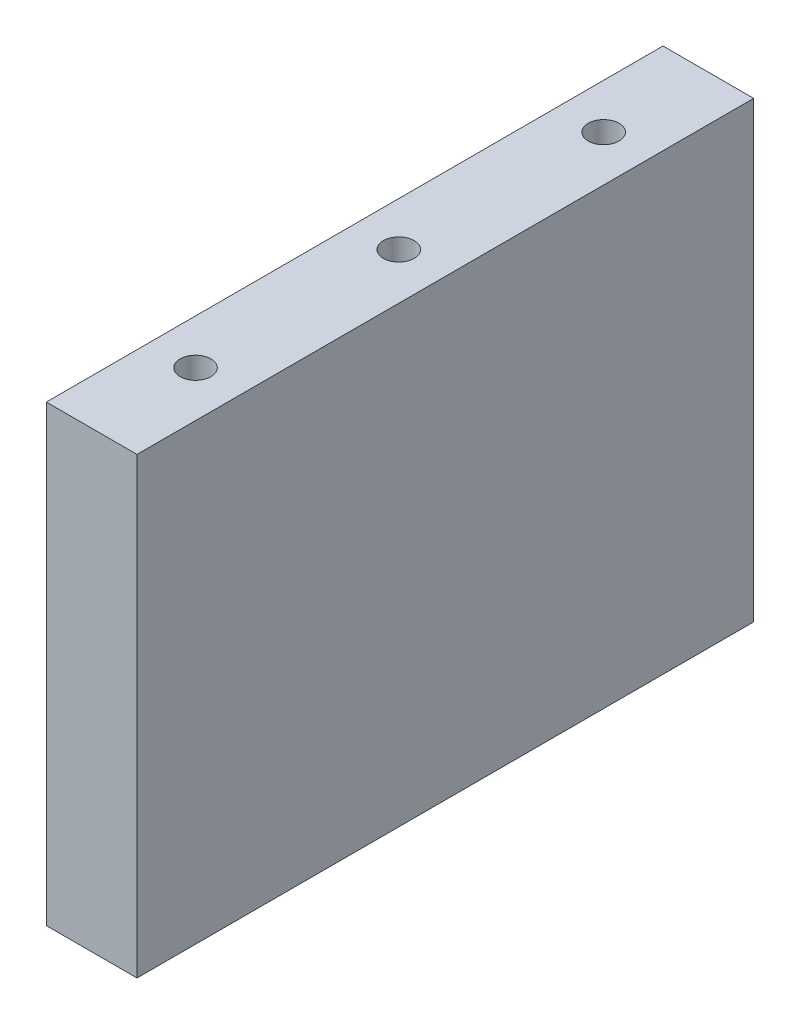
SolidWorks part; units mm, degrees
ref_plane "前视基准面" through (0, 0, 0) normal (0, 0, 1) x (1, 0, 0)
ref_plane "上视基准面" through (0, 0, 0) normal (0, 1, 0) x (1, 0, 0)
ref_plane "右视基准面" through (0, 0, 0) normal (1, 0, 0) x (0, 0, -1)
sketch "草图1" plane through (0, 0, 0) normal (1, 0, 0) x (0, 0, -1)
  line L1 (-68, 50) -> (68, 50)
  line L2 (-68, 50) -> (-68, -50)
  line L3 (-68, -50) -> (68, -50)
  line L4 (68, 50) -> (68, -50)
  line L5 (-68, 50) -> (68, -50) construction
  line L6 (-68, -50) -> (68, 50) construction
  point P0 (0, 0)
  dimension "D1" = 136
  dimension "D2" = 100
extrude "凸台-拉伸1" add sketch "草图1" along normal blind 20
hole_wizard "M8 螺纹孔1" positions "草图2" profile "草图3" tap size "M8" standard "GB"
sketch "草图2" plane through (0, 50, 0) normal (0, 1, 0) x (1, 0, 0)
  line L0 (0, 0) -> (31.5986, 0) construction
  line L2 (10, -68) -> (9.5475, 47.828) construction
  line L3 (20, -68) -> (0, -68) construction
  point P0 (9.9101, 45)
  point P2 (9.9101, -45)
  point P15 (9.7343, 0)
  dimension "D1" = 90
sketch "草图3" plane through (9.9101, 50, -45) normal (1, 0, 0) x (0, 0, 1)
  line L0 (0, 0) -> (0, 21.7929)
  line L1 (0, 21.7929) -> (3.4, 19.75)
  line L2 (3.4, 19.75) -> (3.4, 0)
  line L5 (3.4, 0) -> (0, 0)
  line L10 (0, 21.7929) -> (-3.4, 19.75) construction
  line L11 (0, -6.35) -> (0, 107.95) construction
  dimension "螺纹孔钻头直径" = 6.8
  dimension "螺纹孔钻头深度" = 19.75
  dimension "导头角度" = 118
cosmetic thread "孔螺蚊线1" parameters "D1"=16, "D2"=8
cosmetic thread "孔螺蚊线2" parameters "D1"=16, "D2"=8
cosmetic thread "孔螺蚊线6" parameters "D1"=16, "D2"=8
hole_wizard "M8 螺纹孔2" positions "草图4" profile "草图5" tap size "M8" standard "GB"
sketch "草图4" plane through (0, -50, 0) normal (0, -1, 0) x (-1, 0, 0)
  line L0 (-10, -68) -> (-10, 27.3351) construction
  line L1 (-20, -68) -> (0, -68) construction
  line L3 (0, 0) -> (-33.0288, 0) construction
  point P0 (-10, 45)
  point P2 (-10, 0)
  point P4 (-10, -45)
  dimension "D1" = 90
sketch "草图5" plane through (10, -50, -45) normal (1, 0, 0) x (0, 0, -1)
  line L0 (0, 0) -> (0, 21.7929)
  line L1 (0, 21.7929) -> (3.4, 19.75)
  line L2 (3.4, 19.75) -> (3.4, 0)
  line L5 (3.4, 0) -> (0, 0)
  line L10 (0, 21.7929) -> (-3.4, 19.75) construction
  line L11 (0, -6.35) -> (0, 107.95) construction
  dimension "螺纹孔钻头直径" = 6.8
  dimension "螺纹孔钻头深度" = 19.75
  dimension "导头角度" = 118
cosmetic thread "孔螺蚊线3" parameters "D1"=16, "D2"=8
cosmetic thread "孔螺蚊线4" parameters "D1"=16, "D2"=8
cosmetic thread "孔螺蚊线5" parameters "D1"=16, "D2"=8
